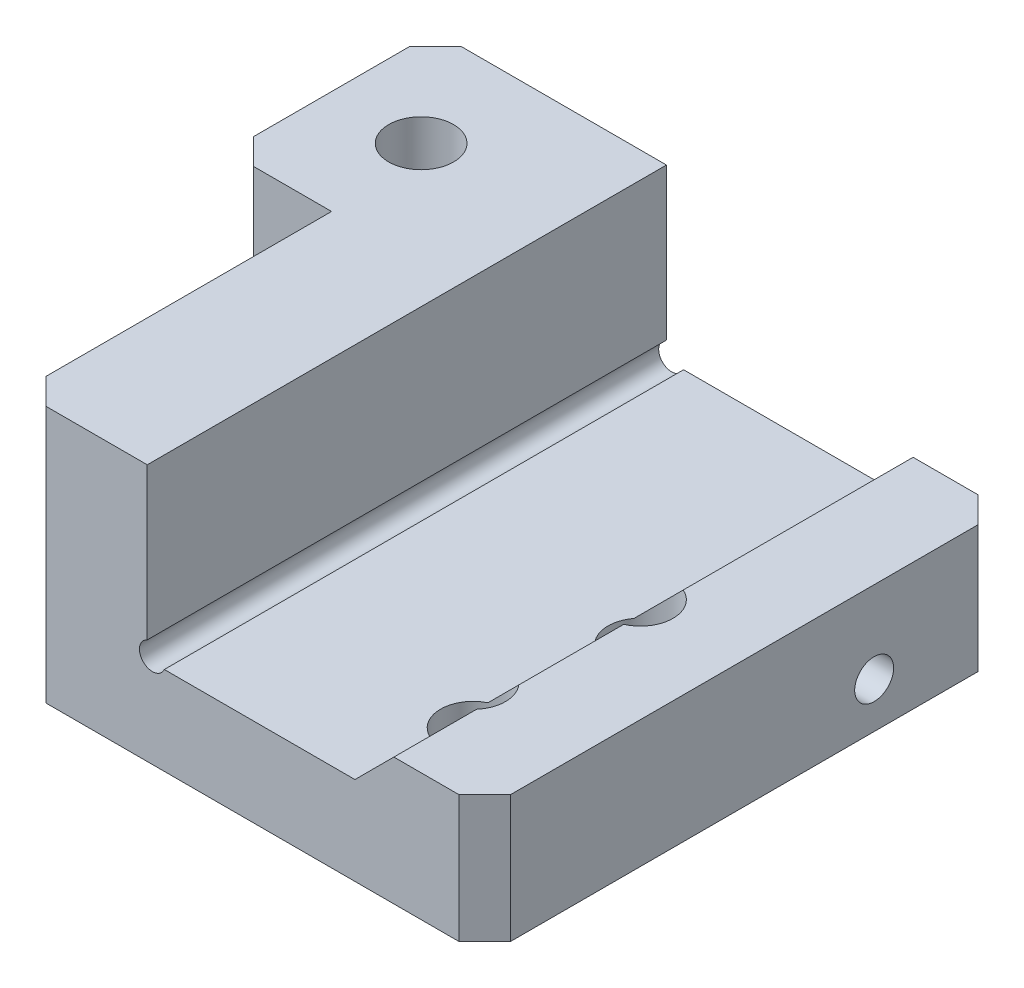
from build123d import *

# Parameters (mm, degrees)
BOSS_EXTRUDE1_DEPTH        = 20
MOVE_FACE1_BY              = 3.4
MOVE_FACE2_BY              = 9.9
BOSS_EXTRUDE2_DEPTH        = 20
M3_TAPPED_HOLE1_D          = 2.5
M3_TAPPED_HOLE1_DEPTH      = 10
M3_TAPPED_HOLE1_TIP        = 0.751075774
SKETCH13_W                 = 4
SKETCH13_H                 = 8
BOSS_EXTRUDE3_DEPTH        = 9.9
M3_TAPPED_HOLE2_D          = 2.5
M3_TAPPED_HOLE2_DEPTH      = 10
M3_TAPPED_HOLE2_TIP        = 0.751075774
CHAMFER1_SIZE              = 1
SIZE_MM_DOWEL_HOLE_0_D     = 1.5
SIZE_MM_DOWEL_HOLE_0_DEPTH = 6
SIZE_MM_DOWEL_HOLE_0_TIP   = 0.450645464


with BuildPart() as part:
    # Sketch1 → Boss-Extrude1 (new body)
    with BuildSketch(Plane.XY):
        with BuildLine():
            Line((0, 0), (0, 6.5))
            Line((0, 6.5), (4.9, 6.5))
            Line((4.9, 6.5), (4.9, 4.058257569))
            ThreePointArc((4.9, 4.058257569), (4.746446609, 3.246446609), (5.558257569, 3.4))
            Line((5.558257569, 3.4), (8, 3.4))
            Line((8, 3.4), (8, 0))
            Line((8, 0), (0, 0))
        make_face()
    extrude(amount=BOSS_EXTRUDE1_DEPTH)

    # Move Face1: a face moved outward by 3.4
    extrude(part.faces().sort_by_distance((2.45, 6.5, 10))[0], amount=MOVE_FACE1_BY, dir=(0, 1, 0))

    # Move Face2: a face moved outward by 9.9
    extrude(part.faces().sort_by_distance((8, 1.7, 10))[0], amount=MOVE_FACE2_BY, dir=(1, 0, 0))

    # Sketch10 → Boss-Extrude2 (add)
    with BuildSketch(Plane(origin=(0, 0, 0), x_dir=(-1, 0, 0), z_dir=(0, 0, -1))):
        Polygon((-17.9, 3.4), (-17.9, 4.9), (-14.4, 4.9), (-12.9, 3.4), align=None)
    extrude(amount=-BOSS_EXTRUDE2_DEPTH)

    # M3 Tapped Hole1
    with Locations(Plane(origin=(0, 0, 0), x_dir=(-1, 0, 0), z_dir=(0, -1, 0))):
        with Locations((-13.9, -10)):
            Hole(M3_TAPPED_HOLE1_D / 2, depth=M3_TAPPED_HOLE1_DEPTH)
            with Locations((0, 0, -(M3_TAPPED_HOLE1_DEPTH + M3_TAPPED_HOLE1_TIP / 2))):  # 118° drill point
                Cone(0, M3_TAPPED_HOLE1_D / 2, M3_TAPPED_HOLE1_TIP, mode=Mode.SUBTRACT)

    # Sketch13 → Boss-Extrude3 (add)
    with BuildSketch(Plane.XZ):
        with Locations((-2, 4)):
            Rectangle(SKETCH13_W, SKETCH13_H)
    extrude(amount=-BOSS_EXTRUDE3_DEPTH)

    # M3 Tapped Hole2
    with Locations(Plane(origin=(0, 0, 0), x_dir=(-1, 0, 0), z_dir=(0, -1, 0))):
        with Locations((-13.45, -16), (0.55, -4)):
            Hole(M3_TAPPED_HOLE2_D / 2, depth=M3_TAPPED_HOLE2_DEPTH)
            with Locations((0, 0, -(M3_TAPPED_HOLE2_DEPTH + M3_TAPPED_HOLE2_TIP / 2))):  # 118° drill point
                Cone(0, M3_TAPPED_HOLE2_D / 2, M3_TAPPED_HOLE2_TIP, mode=Mode.SUBTRACT)

    # Chamfer1
    chamfer1_edges = [part.edges().sort_by_distance(p)[0] for p in [
        (0, 4.95, 20),
        (-4, 4.95, 0),
        (-4, 4.95, 8),
        (17.9, 2.45, 20),
        (17.9, 2.45, 0),
    ]]
    chamfer(chamfer1_edges, length=CHAMFER1_SIZE)

    # Size mm dowel hole 0
    with Locations(Plane(origin=(17.9, 0, 0), x_dir=(0, 0, -1), z_dir=(1, 0, 0))):
        with Locations((-5, 1.75)):
            Hole(SIZE_MM_DOWEL_HOLE_0_D / 2, depth=SIZE_MM_DOWEL_HOLE_0_DEPTH)
            with Locations((0, 0, -(SIZE_MM_DOWEL_HOLE_0_DEPTH + SIZE_MM_DOWEL_HOLE_0_TIP / 2))):  # 118° drill point
                Cone(0, SIZE_MM_DOWEL_HOLE_0_D / 2, SIZE_MM_DOWEL_HOLE_0_TIP, mode=Mode.SUBTRACT)


solid = part.part
